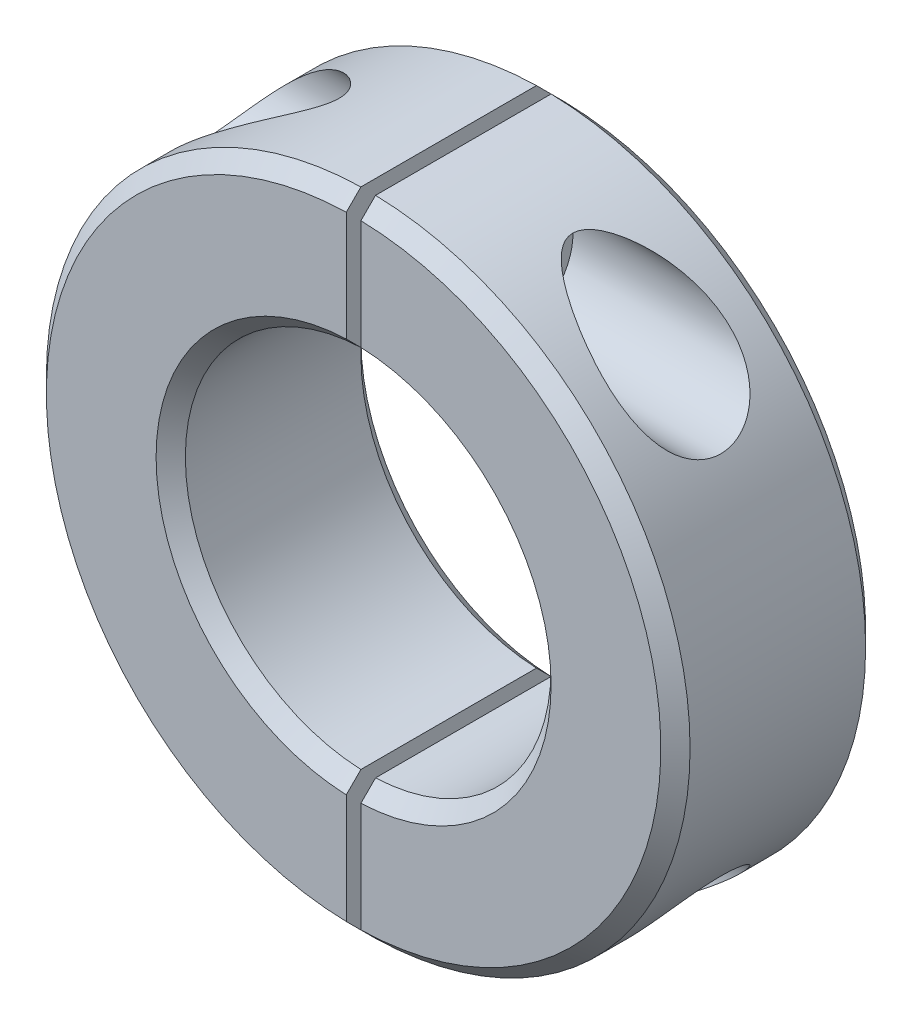
from build123d import *

# Parameters (mm, degrees)
EXTRUDE_1_DEPTH     = 7
CHAMFER_1_SIZE      = 1
SKETCH_2_W          = 1
SKETCH_2_H          = 75.347210032
CUT_EXTRUDE_1_DEPTH = 35.117444218
SKETCH_3_R          = 4
CUT_EXTRUDE_2_DEPTH = 30.270292107
CUT_EXTRUDE_3_REACH = 31.27
SKETCH_4_R          = 2.5


with BuildPart() as part:
    # 草图1 → 凸台-拉伸1 (new, symmetric)
    with BuildSketch(Plane.XY):
        with BuildLine():
            Line((0, 22), (0, 12.5))
            ThreePointArc((0, 12.5), (12.5, 0), (0, -12.5))
            Line((0, -12.5), (0, -22))
            ThreePointArc((0, -22), (22, 0), (0, 22))
        make_face()
    extrude(amount=EXTRUDE_1_DEPTH, both=True)

    # 倒角1
    chamfer_1_edges = [part.edges().sort_by_distance(p)[0] for p in [
        (12.5, 0, 7),
        (22, 0, 7),
        (12.5, 0, -7),
        (22, 0, -7),
    ]]
    chamfer(chamfer_1_edges, length=CHAMFER_1_SIZE)

    # 草图2 → 切除-拉伸1 (cut, through all)
    with BuildSketch(Plane.XY.offset(7)):
        Rectangle(SKETCH_2_W, SKETCH_2_H)
    extrude(amount=-CUT_EXTRUDE_1_DEPTH, mode=Mode.SUBTRACT)

    # 草图3 → 切除-拉伸2 (cut, through all)
    with BuildSketch(Plane(origin=(4, 0, 0), x_dir=(0, 0, -1), z_dir=(1, 0, 0))):
        with Locations(Location((0, -16.5, 0), (0, 0, 180))):
            Circle(SKETCH_3_R)
        with Locations(Location((0, 16.5, 0), (0, 0, 180))):
            Circle(SKETCH_3_R)
    extrude(amount=CUT_EXTRUDE_2_DEPTH, mode=Mode.SUBTRACT)

    # 草图4 → 切除-拉伸3 (cut, up to next)
    with BuildSketch(Plane(origin=(4, 0, 0), x_dir=(0, 0, -1), z_dir=(1, 0, 0)), mode=Mode.PRIVATE) as cut_extrude_3_sk1:
        with Locations((0, 16.5)):
            Circle(SKETCH_4_R)
    cut_extrude_3_tool1 = extrude(cut_extrude_3_sk1.sketch, amount=-CUT_EXTRUDE_3_REACH, mode=Mode.PRIVATE) & part.part
    # 草图4 → 切除-拉伸3 (cut, up to next)
    with BuildSketch(Plane(origin=(4, 0, 0), x_dir=(0, 0, -1), z_dir=(1, 0, 0)), mode=Mode.PRIVATE) as cut_extrude_3_sk2:
        with Locations((0, -16.5)):
            Circle(SKETCH_4_R)
    cut_extrude_3_tool2 = extrude(cut_extrude_3_sk2.sketch, amount=-CUT_EXTRUDE_3_REACH, mode=Mode.PRIVATE) & part.part
    add(cut_extrude_3_tool1.solids().sort_by_distance((4, 16.5, 0))[0], mode=Mode.SUBTRACT)
    add(cut_extrude_3_tool2.solids().sort_by_distance((4, -16.5, 0))[0], mode=Mode.SUBTRACT)


with BuildPart() as body_2:
    # 镜向5: mirrored copy
    add(part.part.mirror(Plane(origin=(0, 0, 0), x_dir=(0, 0, 1), z_dir=(1, 0, 0))))


solid = Compound([part.part, body_2.part])
